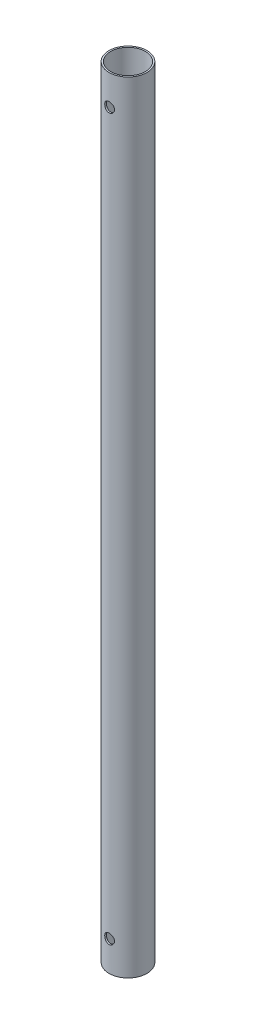
from build123d import *

# Parameters (mm, degrees)
SKETCH_1_R               = 6
SKETCH_1_R_2             = 5.5
EXTRUDE_1_DEPTH          = 246.5
CUT_EXTRUDE_1_DEPTH      = 247.646001387
CUT_EXTRUDE_1_DEPTH_BACK = 247.646001387
SKETCH_2_R               = 1.55


with BuildPart() as part:
    # 草图1 → 凸台-拉伸1 (new body)
    with BuildSketch(Plane(origin=(0, 0, 0), x_dir=(1, 0, 0), z_dir=(0, 1, 0))):
        with Locations(Location((0, 0, 0), (0, 0, 270))):
            Circle(SKETCH_1_R)
        with Locations(Location((0, 0, 0), (0, 0, 270))):
            Circle(SKETCH_1_R_2, mode=Mode.SUBTRACT)
    extrude(amount=EXTRUDE_1_DEPTH)

    # 草图2 → 切除-拉伸1 (cut, two sides: drawn at the far end of the back side and taken through both)
    with BuildSketch(Plane.XY.offset(-CUT_EXTRUDE_1_DEPTH_BACK)):
        with Locations((0, 237)):
            Circle(SKETCH_2_R)
        with Locations((0, 9.5)):
            Circle(SKETCH_2_R)
    extrude(amount=CUT_EXTRUDE_1_DEPTH + CUT_EXTRUDE_1_DEPTH_BACK, mode=Mode.SUBTRACT)


solid = part.part
